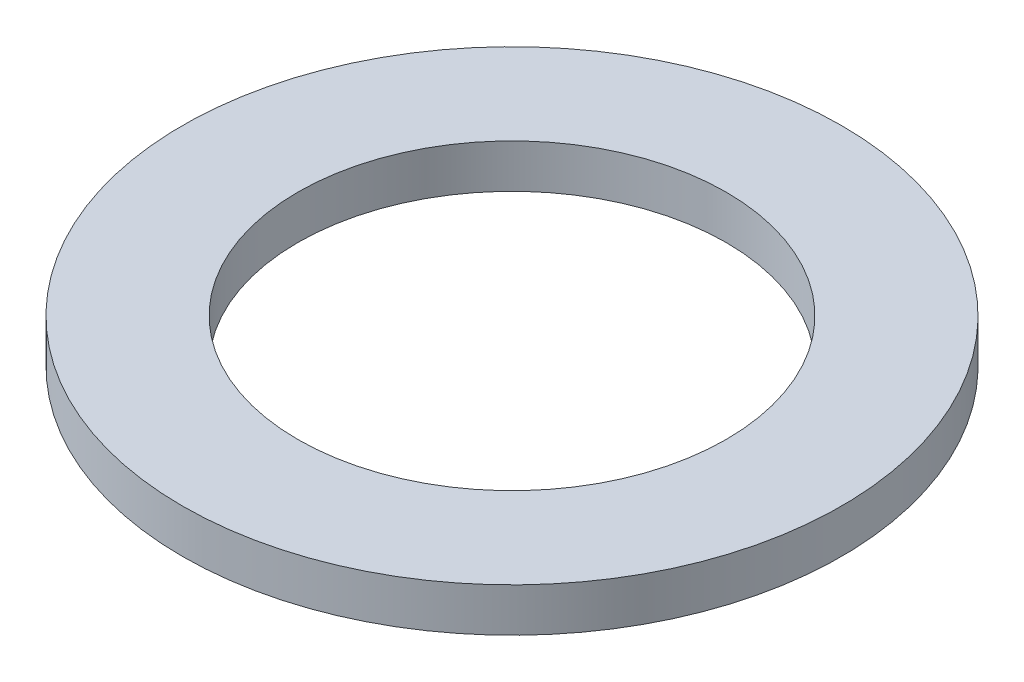
from build123d import *

# Parameters (mm, degrees)
SKETCH1_R           = 40
SKETCH1_R_2         = 26
BOSS_EXTRUDE1_DEPTH = 5.3


with BuildPart() as part:
    # Sketch1 → Boss-Extrude1 (new body)
    with BuildSketch(Plane(origin=(0, 0, 0), x_dir=(1, 0, 0), z_dir=(0, 1, 0))):
        with Locations(Location((0, 0, 0), (0, 0, 270))):
            Circle(SKETCH1_R)
        with Locations(Location((0, 0, 0), (0, 0, 270))):
            Circle(SKETCH1_R_2, mode=Mode.SUBTRACT)
    extrude(amount=BOSS_EXTRUDE1_DEPTH)


solid = part.part
